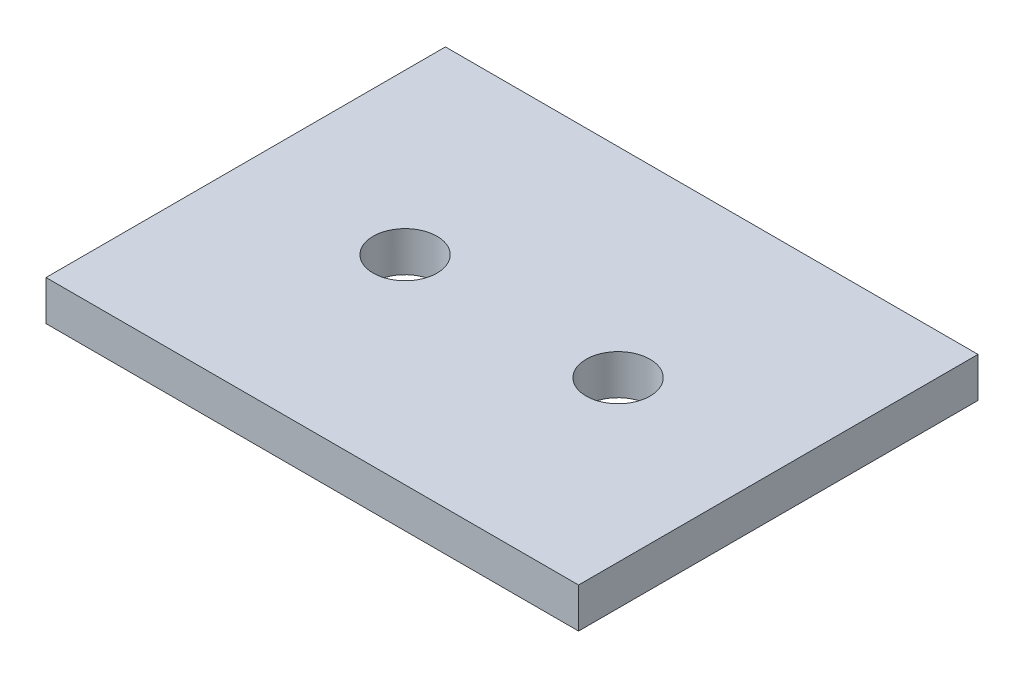
SolidWorks part; units mm, degrees
ref_plane "Front Plane" through (0, 0, 0) normal (0, 0, 1) x (1, 0, 0)
ref_plane "Top Plane" through (0, 0, 0) normal (0, 1, 0) x (1, 0, 0)
ref_plane "Right Plane" through (0, 0, 0) normal (1, 0, 0) x (0, 0, -1)
sketch "Sketch1" plane through (0, 0, 0) normal (0, 1, 0) x (1, 0, 0)
  line L1 (-20, 15) -> (20, 15)
  line L2 (-20, 15) -> (-20, -15)
  line L3 (-20, -15) -> (20, -15)
  line L4 (20, 15) -> (20, -15)
  line L5 (-20, 15) -> (20, -15) construction
  line L6 (-20, -15) -> (20, 15) construction
  point P0 (0, 0)
  dimension "D1" = 40
  dimension "D2" = 30
extrude "Boss-Extrude1" add sketch "Sketch1" along normal blind 3
sketch "Sketch2" plane through (0, 0, 0) normal (0, -1, 0) x (1, 0, 0)
  point P0 (-8, 0.0309)
  point P1 (8, 0.0309)
hole_wizard "M4 Clearance Hole1" positions "3DSketch1" profile "Sketch3" hole size "M4" standard "GB"
sketch3d "3DSketch1"
  point P0 (-8, 0, 0.0309)
  point P3 (8, 0, 0.0309)
sketch "Sketch3" plane through (-8, 0, 0.0309) normal (1, 0, 0) x (0, 0, -1)
  line L0 (0, 0) -> (0, 11.5421)
  line L1 (0, 11.5421) -> (2.4, 10.1)
  line L2 (2.4, 10.1) -> (2.4, 0)
  line L5 (2.4, 0) -> (0, 0)
  line L10 (0, 11.5421) -> (-2.4, 10.1) construction
  line L11 (0, -6.35) -> (0, 107.95) construction
  dimension "孔直径" = 4.8
  dimension "孔深度" = 10.1
  dimension "导头角度" = 118
